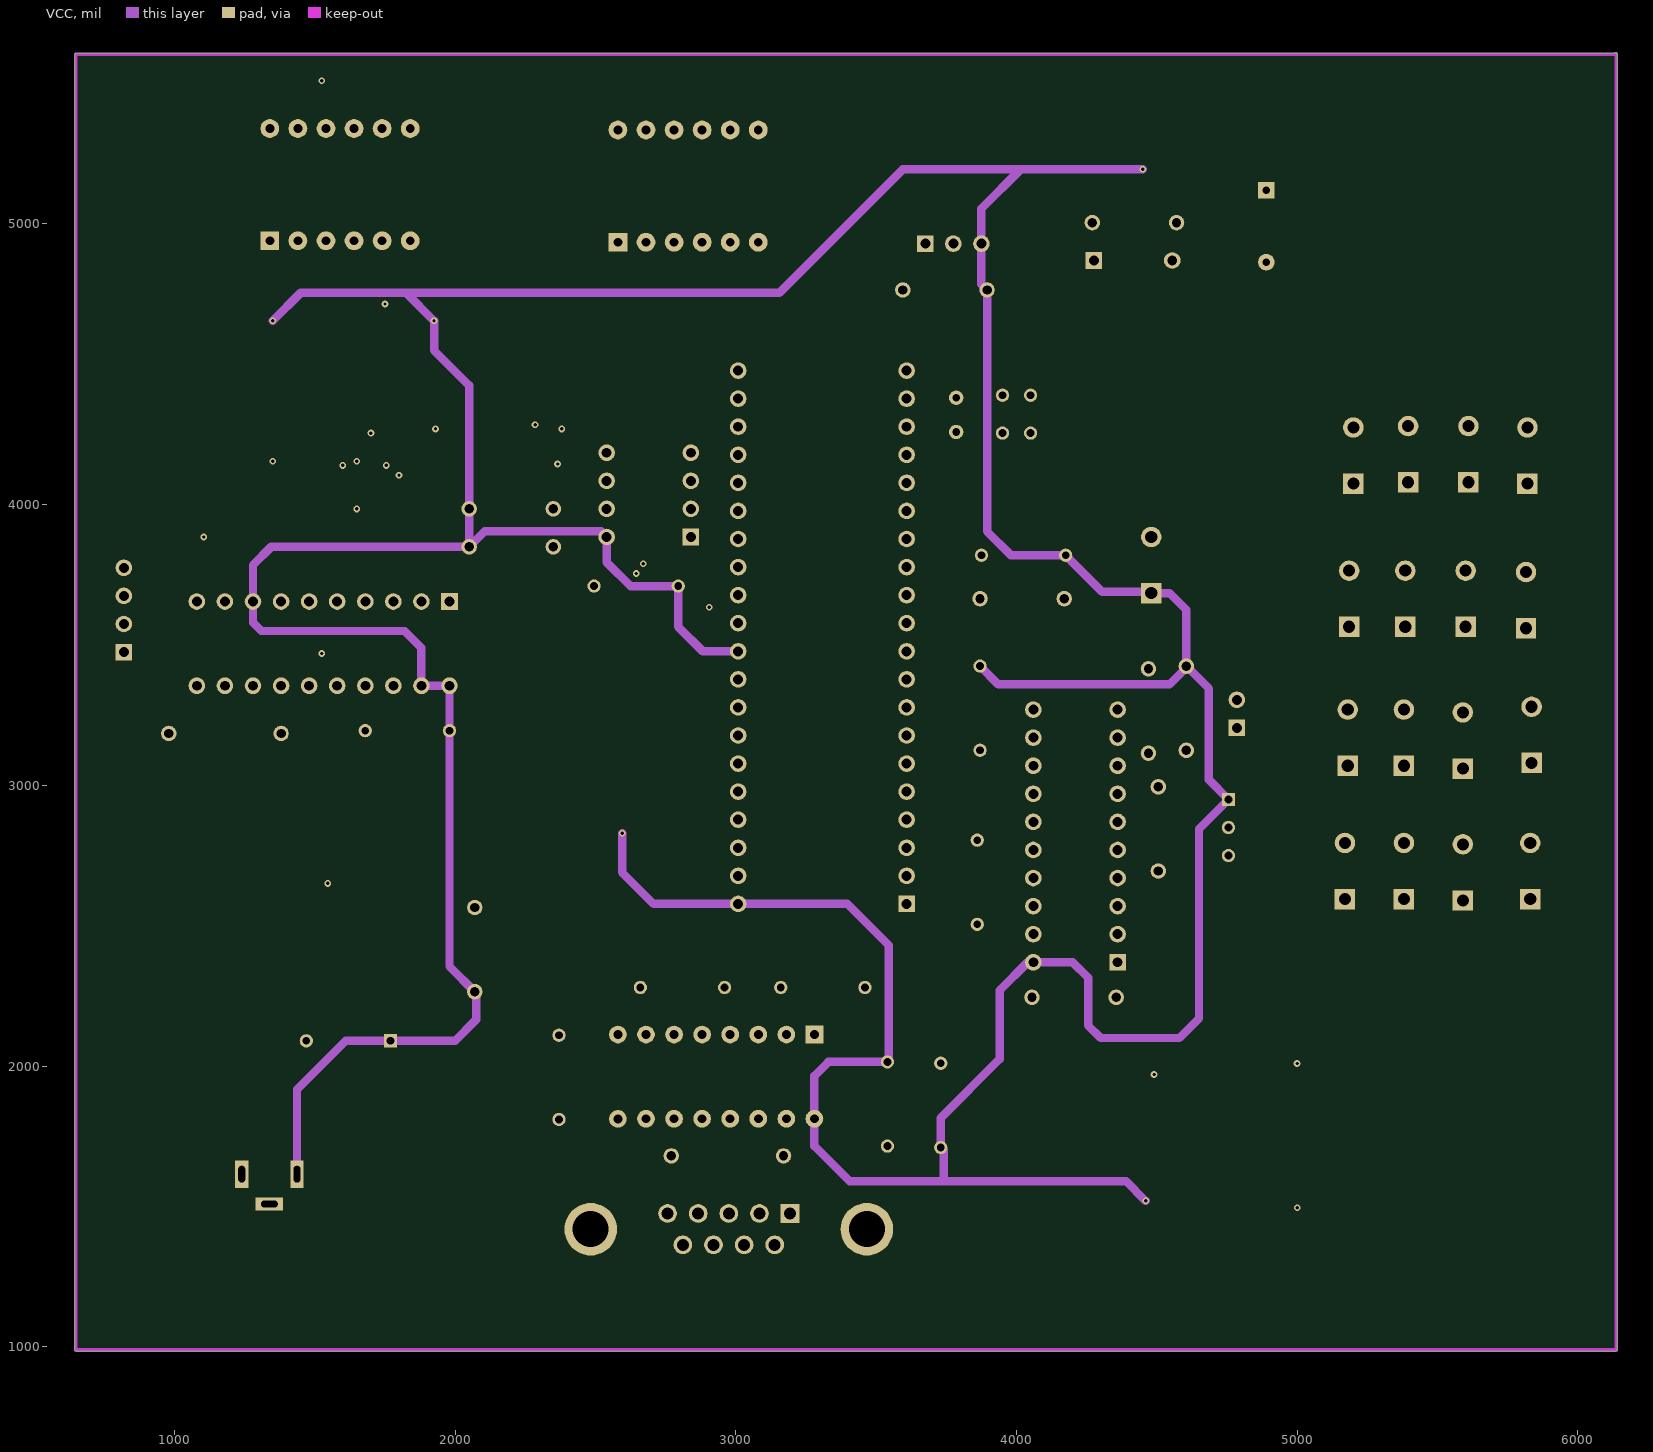
[diagram p0: VCC]
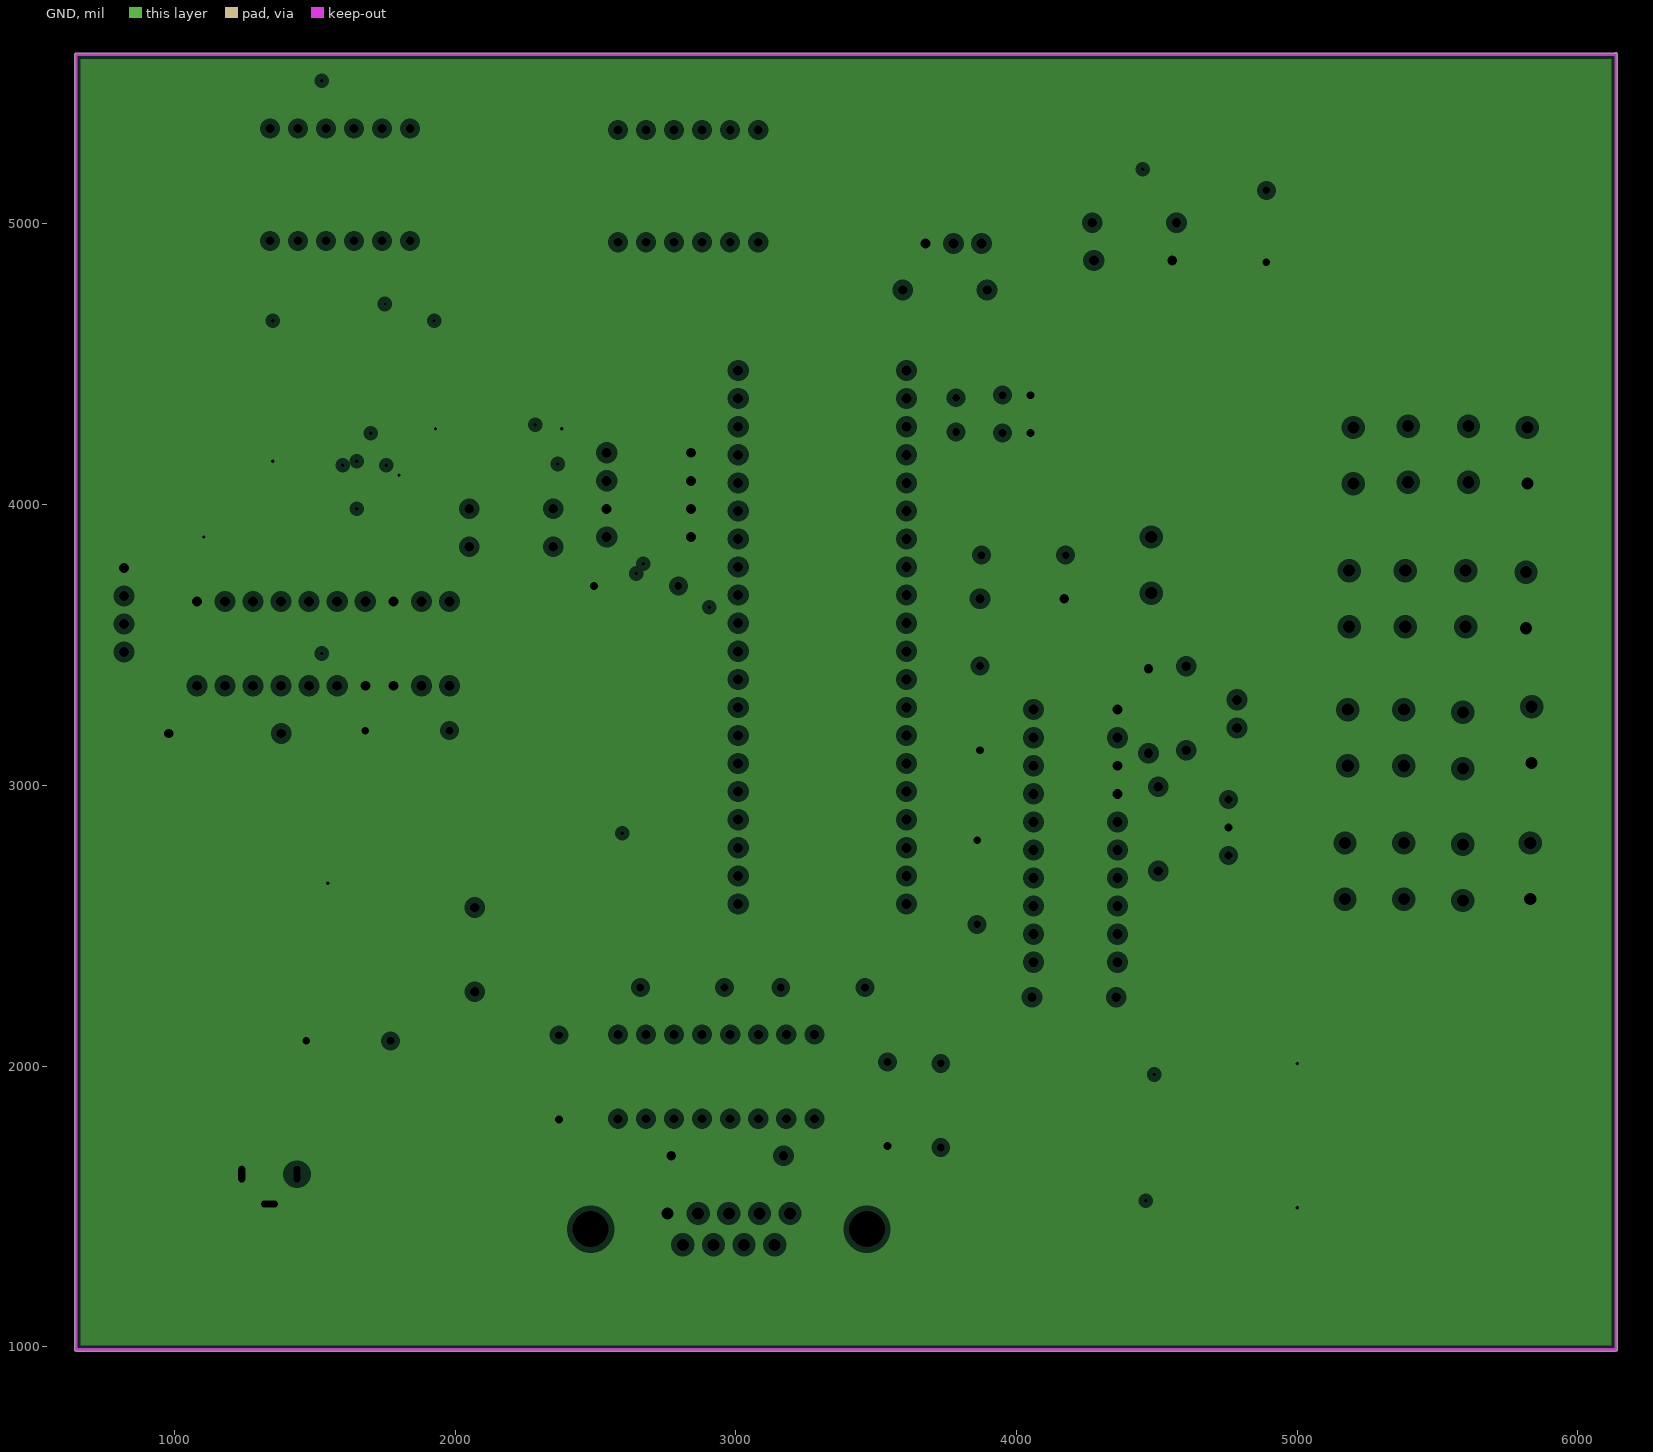
[diagram p1: GND, clearances drawn from the general rule]
# Altium PCB MISC82251.PcbDoc (part 2 of 2)
## Nets (pads, with @x,y where several pads share a name; then routed paths per layer and width w, separated by ;. In a path a pad name is that pad's centre, name@x,y a point inside that pad or via, vN(x,y) a via of type N, cw(c..) or ccw(c..) an arc to the next point about the centre after c; other vN are vias at no path point) (continued)
D0: R8.1 U3.2 U4.2 U5.39 U6.7 | length 3957.8
  Top Layer w10: U4.2 1980,4345 1950,4375 1425,4375 1400,4350 U3.2 1400,3675 U6.7 1380,3445 1430,3395 1430,2990 1645,2775 2620,2775 2705,2860 R8.1 2855,2860 2895,2820 2895,2730 2947.24,2677.76 U5.39
D1: R8.2 U3.3 U4.3 U5.38 U6.6 | length 3717.6
  Top Layer w10: U4.3 2030,4145 2005,4120 1915,4120 1890,4145 1890,4295 1845,4340 1475,4340 1450,4315 U3.3 1450,3685 U6.6 1480,3570 1555,3495 2496.72,3495 2655,3336.72 2655,2970 2715,2910 R8.2 2915,2910 2940,2885 2940,2810 2965,2785 3001.28,2785 U5.38
D2: R8.3 U3.4 U4.4 U5.37 U6.5 | length 3529.2
  Top Layer w10: U4.4 2080,4140 2035,4095 1911.72,4095 1865,4141.72 1865,4290 1845,4310 1525,4310 1500,4285 U3.4 1500,3735 U6.5 1580,3565 1630,3515 2505,3515 2675,3345 2675,2990 2705,2960 R8.3 2926.28,2960 U5.37
D3: R8.4 U3.5 U4.5 U5.36 U6.4 | length 3365.6
  Top Layer w10: U4.5 2130,4135 2065,4070 1895,4070 1845,4120 1845,4270 1830,4285 1570,4285 1550,4265 U3.5 1550,3785 U6.4 1680,3610 1745,3545 2520,3545 2695,3370 2695,3030 2715,3010 R8.4 2976.28,3010 U5.36
D4: R8.5 U3.6 U4.6 U5.35 U6.16 | length 3550.8
  Top Layer w10: v1(1525,3470) 1525,3455 1580,3400 U6.16 ; U3.6 v1(1600,4140) 1700,4040 2115,4040 2180,4105 U4.6 ; R8.5 2990.77,3060 U5.35
  Bottom Layer w10: v1(1525,3470) 1525,4065 v1(1600,4140) ; U6.16 1580,3170 1672.24,3077.76 U5.35
D5: R8.6 U3.7 U4.7 U5.34 U6.15 | length 3531.8
  Top Layer w10: v1(1650,3985) 1690,3945 2029.81,3945 2032.37,3942.44 2132.44,3942.44 2230,4040 U4.7 ; v1(1650,4155) U3.7 ; R8.6 2870,3110 2937.76,3177.76 U5.34
  Bottom Layer w10: U6.15 1480,3375 1535,3430 1635,3430 ; v1(1650,4155) v1(1650,3985) 1650,3725 1630,3705 1630,3435 1635,3430 ; U5.34 2756.28,3430 1635,3430
D6: R8.7 U3.8 U4.8 U5.33 U6.14 | length 4326.4
  Top Layer w10: v1(2285,4285) 2280,4280 U4.8 2280,3810 2455,3635 2625,3635 2715,3545 2715,3204.56 2759.56,3160 R8.7 2850,3160 2875,3185 2875,3230 2922.76,3277.76 U5.33
  Bottom Layer w10: U6.14 1380,3475 1360,3495 1080,3495 1010,3565 1010,4235 1085,4310 1720,4310 ; v1(1700,4255) 1700,4290 1720,4310 ; v1(2285,4285) 2260,4310 1720,4310
D7: R8.8 U3.9 U4.9 U5.32 U6.13 | length 3811.7
  Top Layer w10: U3.9 1750,4145 v1(1755,4140) ; U4.9 2330,4180 v1(2365,4145) 2420,4090 2420,3705 2470,3655 2685,3655 2778.98,3561.02 R8.8 2835,3210 2855,3230 2855,3360 2872.76,3377.76 U5.32
  Bottom Layer w10: U6.13 1280,3295 1300,3275 1415,3275 1430,3290 1430,4115 1515,4200 1705,4200 1755,4150 v1(1755,4140) 2360,4140 v1(2365,4145)
DB1: U2.18 U5.1 U8.19 | length 1908.2
  Top Layer w10: U5.1 4052.24,2577.76 U2.18 4120,2510 4120,1690 4235,1575 U8.19
DB2: U2.17 U5.2 U8.18 | length 1931.8
  Top Layer w10: U5.2 4052.24,2677.76 U2.17 4140,2590 4140,1765 4280,1625 U8.18
DB3: U2.16 U5.3 U8.17 | length 2044.1
  Top Layer w10: U5.3 3631.28,2755 4045,2755 U2.16 4145,2770 4165,2750 4165,1790 4280,1675 U8.17
DB4: U2.15 U5.4 U8.16 | length 2081.6
  Top Layer w10: U5.4 4052.24,2877.76 U2.15 4150,2870 4185,2835 4185,1825 4285,1725 U8.16
DB5: U2.14 U5.5 U8.15 | length 2140.4
  Top Layer w10: U5.5 3616.28,2970 U2.14 4180,2970 4205,2945 4205,1870 4300,1775 U8.15
DB6: U2.13 U5.6 U8.14 | length 2146.5
  Top Layer w10: U5.6 4052.24,3077.76 U2.13 4190,3070 4225,3035 4225,1985 4385,1825 U8.14
DB7: U2.12 U5.7 U8.13 | length 2214.1
  Top Layer w10: U5.7 3616.28,3170 U2.12 4220,3170 4245,3145 4245,2015 4385,1875 U8.13
DB8: U2.11 U5.8 U8.12 | length 2255.3
  Top Layer w10: U5.8 4052.24,3277.76 U2.11 4215,3270 4285,3200 4285,2035 4395,1925 U8.12
DCDEN: U5.14
DIOLA: U5.26 U8.11 | length 3427.4
  Top Layer w10: v1(4490,1970) 4495,1975 U8.11
  Bottom Layer w10: U5.26 3242.24,3977.76 3315,3905 3315,2415 3385,2345 3780,2345 3840,2285 3840,2100 3895,2045 4415,2045 v1(4490,1970)
DP: SMG1.3 SMG2.3 U3.12 | length 2007.4
  Top Layer w10: U3.12 v1(1750,4715)
  Bottom Layer w10: v1(1750,4715) 1750,4775 1715,4810 1575,4810 1540,4845 SMG1.3 1540,4990 1605,5055 2175,5055 2390,4840 2755,4840 2780,4865 SMG2.3
DULA: U3.11 U5.27 | length 1981.3
  Top Layer w10: U3.11 1800,4475 1850,4425 2615,4425 2655,4385 2655,3805 v1(2670,3790)
  Bottom Layer w10: v1(2670,3790) 2920.77,3790 U5.27
E: SMG1.1 SMG2.1 U3.15 | length 2088.7
  Top Layer w10: SMG1.1 1340,4795 1360,4775 1535,4775 1600,4710 U3.15
  Bottom Layer w10: SMG1.1 1340,5075 1375,5110 2515,5110 2580,5045 SMG2.1
F: SMG1.10 SMG2.10 U3.14 | length 4045
  Top Layer w10: v1(1525,5510) 1055,5510 975,5430 975,4545 1045,4475 1605,4475 1650,4520 U3.14
  Bottom Layer w10: v1(1525,5510) 1540,5495 SMG1.10 1540,5260 1575,5225 2415,5225 2450,5260 2450,5420 2480,5450 2735,5450 2780,5405 SMG2.10
G: SMG1.5 SMG2.5 U3.13 | length 1863.2
  Top Layer w10: U3.13 1700,4900 SMG1.5
  Bottom Layer w10: SMG1.5 1805,5005 2125,5005 2350,4780 2945,4780 2980,4815 SMG2.5
GND: C1.1 C4.1 C5.2 C7.1 C8.2 C10.2 C11.2 C12.2 C13.2 D1.2 D2.2 D3.1 J1.5 J2.2 J2.3 LS1.2 LS1.2A P1.1 P3.4 R1.2 R5.1 R7.2 R9.2 R10.1 S2.1 S7.1 S12.1 S17.1 U2.7 U2.8 U2.10 U3.1 U3.10 U4.1 U4.10 U6.3 U6.10 U6.17 U6.18 U7.1 U7.2 U7.3 U7.4 U7.7 U8.1 U8.10 | length 535
  Top Layer w30: D1.2 1099.06,3879.06 v1(1105,3885) ; v1(1350,4155) U3.1 ; D2.2 v1(1545.94,2650.94) v1@1550,2655 ; v1(1800,4105) U3.10 ; U4.1 v1(1930,4270) ; U4.10 v1@2380,4275 ; U8.1 4998.98,1496.02 v1(5000,1495) ; U8.10 4998.98,2008.98 v1@5000,2010
  other v1: 4999.49,2009.49 2380,4270
INT0: S13.1 S14.1 S15.1 S16.1 U5.12 U6.1 | length 5741.9
  Top Layer w10: v1(2905,3635) 2906.77,3633.23 3564,3633.23 U5.12 ; S13.1 5695,2695 5695,2970 ; S14.1 5680,2970 5695,2970 ; S15.1 5685,3565 5695,3555 ; S16.1 5695,3995 5695,3555 ; 5695,2970 5695,3555
  Bottom Layer w10: U6.1 2885,3655 v1(2905,3635) ; U5.12 4140.77,4210 5480,4210 S16.1
INT1: U5.13
LCDEN: S2.2 S3.2 S8.2 S13.2 | length 660
  Bottom Layer w10: S3.2 S8.2 S2.2
M11: SMG1.12 U4.19 | length 1345.2
  Top Layer w10: SMG1.12 1340,5150 1380,5110 1940,5110 1980,5070 U4.19
M12: SMG1.9 U4.18 | length 1048.3
  Top Layer w10: SMG1.9 1640,5230 1715,5155 1945,5155 2030,5070 U4.18
M13: SMG1.8 U4.17 | length 1033.5
  Top Layer w10: SMG1.8 1740,5255 1810,5185 2050,5185 2080,5155 U4.17
M21: SMG2.12 U4.16 | length 1138.5
  Top Layer w10: U4.16 2130,5070 2190,5130 2540,5130 2580,5170 SMG2.12
M22: SMG2.9 U4.15 | length 1385.5
  Top Layer w10: U4.15 2180,5020 2240,5080 2835,5080 2880,5125 SMG2.9
M23: SMG2.8 U4.14 | length 1435.5
  Top Layer w10: U4.14 2230,5015 2275,5060 2920,5060 2980,5120 SMG2.8
NetC2_1: C2.1 U1.1 | length 329.9
  Top Layer w10: U1.1 3280,2250 3310,2280 C2.1
NetC2_2: C2.2 U1.3 | length 200.6
  Top Layer w10: U1.3 3080,2200 C2.2
NetC3_2: C3.2 U1.2 | length 725.6
  Top Layer w10: U1.2 3180,2010 3220,1970 3710,1970 3750,2010 C3.2
NetC5_1: C5.1 R2.1 U2.19 | length 664.4
  Top Layer w10: R2.1 3890,2245 3845,2290 3845,2490 C5.1 4025,2505 U2.19
NetC6_1: C6.1 U1.4 | length 220.7
  Top Layer w10: C6.1 2960,2110 2979.99,2090.01 U1.4
NetC6_2: C6.2 U1.5 | length 331.9
  Top Layer w10: C6.2 2785,2280 2880,2185 U1.5
NetC7_2: C7.2 U1.6 | length 567.2
  Top Layer w10: C7.2 2370,2165 2430,2225 2720,2225 2780,2165 U1.6
NetD1_1: D1.1 P3.3 | length 225.6
  Top Layer w10: P3.3 924.06,3675 D1.1
NetD2_1: D2.1 R12.1 | length 408
  Top Layer w10: D2.1 2065,2570 R12.1
NetD3_2: D3.2 LS1.1 LS1.1A Q1.1 | length 1012.1
  Top Layer w10: D3.2 4345,4870 4377.6,4902.6 Q1.1 4377.6,5242.6 4410,5275 4848.78,5275 LS1.1
NetD4_1: D4.1 R15.8 | length 222.1
  Top Layer w10: D4.1 5723.11,1455 R15.8
NetD4_2: D4.2 U8.2 | length 673.3
  Top Layer w10: U8.2 5080,1575 5110,1545 5110,1430 5170,1370 D4.2
NetD5_1: D5.1 R15.7 | length 485.7
  Top Layer w10: D5.1 5685,1455 5735,1505 R15.7
NetD5_2: D5.2 U8.3 | length 386.6
  Top Layer w10: U8.3 5115,1625 5145,1595 5145,1470 5160,1455 D5.2
NetD6_1: D6.1 R15.6 | length 187.1
  Top Layer w10: D6.1 5645,1555 R15.6
NetD6_2: D6.2 U8.4 | length 624.5
  Top Layer w10: U8.4 5140,1675 5165,1650 5165,1565 5180,1550 D6.2
NetD7_1: D7.1 R15.5 | length 479.5
  Top Layer w10: D7.1 5685,1640 5715,1610 5820,1610 R15.5
NetD7_2: D7.2 U8.5 | length 278.1
  Top Layer w10: U8.5 5156.72,1725 5241.72,1640 D7.2
NetD8_1: D8.1 R15.4 | length 213
  Top Layer w10: D8.1 5718.11,1655 R15.4
NetD8_2: D8.2 U8.6 | length 544.7
  Top Layer w10: U8.6 5135,1775 5180,1730 D8.2
NetD9_1: D9.1 R15.3 | length 512.6
  Top Layer w10: D9.1 5665,1820 5780,1705 R15.3
NetD9_2: D9.2 U8.7 | length 245
  Top Layer w10: U8.7 5236.89,1825 D9.2
NetD10_1: D10.1 R15.2 | length 306.7
  Top Layer w10: D10.1 5730,1910 5750,1890 5750,1785 5780,1755 R15.2
NetD10_2: D10.2 U8.8 | length 541.5
  Top Layer w10: U8.8 5185,1875 5220,1910 D10.2
NetD11_1: D11.1 R15.1 | length 669.9
  Top Layer w10: D11.1 5385,2020 5790,2020 5825,1985 R15.1
NetD11_2: D11.2 U8.9 | length 271.9
  Top Layer w10: U8.9 5171.89,1925 D11.2
NetJ1_2: J1.2 U1.14 | length 339.2
  Top Layer w10: U1.14 3080,1479.06 J1.2
NetJ1_3: J1.3 U1.13 | length 339.6
  Top Layer w10: J1.3 2975,1807.5 U1.13
NetP2_1: P2.1 R4.1 R6.2 R7.1 U2.9 | length 619.6
  Top Layer w10: U2.9 4415,3170 R7.1 ; R4.1 4470,3030 R7.1 ; P2.1 4705,3125 R6.2 4595,3115 R7.1
NetP2_2: P2.2 R1.3 | length 804
  Top Layer w10: R1.3 4885,2750 4915,2780 4915,3265 4875,3305 P2.2
NetP3_1: P3.1 U6.9 | length 517.8
  Top Layer w10: P3.1 1135,3475 1185,3525 1185,3650 U6.9
NetP3_2: P3.2 U6.11 | length 563.8
  Top Layer w10: P3.2 740,3495 740,3405 790,3355 U6.11
NetQ1_2: Q1.2 R11.1 | length 196.3
  Top Layer w10: Q1.2 4452.4,5042.6 4480,5015 4560,5015 R11.1
NetR2_2: R2.2 U2.4 | length 460.2
  Top Layer w10: R2.2 4315,2285 4315,2625 U2.4
NetR4_2: R4.2 U2.6 | length 302.4
  Top Layer w10: U2.6 4475,2870 4505,2840 R4.2
NetR5_2: R5.2 U1.15 | length 136.6
  Top Layer w10: R5.2 3180,1690 U1.15
NetR9_1: R9.1 U6.12 | length 334.9
  Top Layer w10: U6.12 1180,3245 1240,3185 R9.1
P30: S3.1 S4.1 S5.1 S6.1 U1.12 U5.10 | length 7202
  Top Layer w10: U1.12 2879.99,1945.01 2820,2005 2375,2005 2290,2090 2290,2310 2365,2385 3225,2385 3310,2470 3310,3385 3402.76,3477.76 U5.10 ; S3.1 5300,2725 5300,3070 ; S4.1 5300,3070 ; S5.1 5290,3565 5300,3555 ; S6.1 5300,3975 5300,3555 ; 5300,3070 5300,3555
  Bottom Layer w10: U5.10 4592.76,3477.76 4775,3660 4775,4015 4835,4075 S6.1
P31: S8.1 S9.1 S10.1 S11.1 U1.11 U5.11 | length 7603.6
  Top Layer w10: U1.11 2780,1885 2720,1945 2320,1945 2235,2030 2235,2360 2310,2435 3105,2435 3175,2505 3175,3470 3282.76,3577.76 U5.11 ; S8.1 5505,2720 5505,3075 ; S9.1 5500,3070 5505,3075 ; S10.1 5505,3565 ; S11.1 5505,3970 5505,3565 ; 5505,3075 5505,3565
  Bottom Layer w10: U5.11 4562.76,3577.76 4685,3700 4685,4120 4745,4180 5295,4180 S11.1
PSEN: U5.29
RD: S6.2 S11.2 S16.2 S17.2 U2.2 U5.17 | length 5460.9
  Top Layer w10: U5.17 5102.76,4177.76 S6.2 5760,4275 5765,4280 5815,4280 S17.2
  Bottom Layer w10: U5.17 3537.76,4177.76 3430,4070 3430,2460 3455,2435 3875,2435 3930,2380 3930,2255 4020,2165 4185,2165 4215,2195 4215,2400 4285,2470 U2.2
RS: S4.2 S7.2 S9.2 S14.2 U5.15 | length 2743.4
  Top Layer w10: U5.15 4757.24,3977.76 5045,3690 5045,3315 5090,3270 S4.2
  Bottom Layer w10: S4.2 S9.2 5825,3270 S7.2
RST: C9.1 R10.2 S1.2 U5.9 | length 1248.5
  Top Layer w10: U5.9 3717.76,3377.76 3870,3530 R10.2 3870,3815 C9.1 3940,3885 S1.2
SCL: R13.1 U5.22 U7.6 | length 903.5
  Bottom Layer w10: R13.1 2440,3940 2440,3985 U7.6 2832.76,4377.76 U5.22
SDA: R14.1 U5.21 U7.5 | length 1009.1
  Bottom Layer w10: R14.1 2455,4090 2455,4100 U7.5 2540,4425 2592.76,4477.76 U5.21
SPK: R11.2 U5.24 | length 1899.9
  Bottom Layer w10: U5.24 3307.76,4177.76 3430,4300 3430,4590 3490,4650 4045,4650 4135,4740 4135,4955 4185,5005 R11.2
VCC: C1.2 C3.1 C4.2 C8.1 C9.2 C10.1 C12.1 J2.1 P1.3 Q1.3 R1.1 R3.2 R6.1 R8.9 R8.10 R8.11 R8.12 R8.13 R8.14 R8.15 R8.16 R12.2 R13.2 R14.2 R15.9 R15.10 R15.11 R15.12 R15.13 R15.14 R15.15 R15.16 S1.1 U1.16 U2.20 U3.20 U4.20 U5.31 U5.40 U6.8 U6.19 U6.20 U7.8 U8.20 | length 22354.1
  Top Layer w30: U3.20 v1(1350,4655) ; v1(1925,4655) 1930,4650 U4.20 ; R8.9 R8.10 R8.11 R8.12 R8.13 R8.14 R8.15 R8.16 2590,2835 v1(2595,2830) ; Q1.3 4449.29,5194.29 v1(4450,5195) ; v1(4460,1520) 4465,1525 U8.20 4621.02,1343.98 4755,1210 5920,1210 6013.98,1303.98 R15.9 R15.10 R15.11 R15.12 R15.13 R15.14 R15.15 R15.16
  VCC w30: v1(1350,4655) 1450,4755 1825,4755 ; J2.1 1436.85,1916.85 1610,2090 C10.1 2000,2090 2075,2165 2075,2260 R12.2 1980,2355 C8.1 U6.20 U6.19 1880,3490 1820,3550 1310,3550 1280,3580 U6.8 1280,3785 1345,3850 R13.2 ; v1(2595,2830) 2595,2690 2707.24,2577.76 U5.40 3397.24,2577.76 3545,2430 3545,2020 C4.2 3329.99,2015 3279.99,1965 U1.16 3279.99,1715.01 3405,1590 3740,1590 ; U5.31 2882.24,3477.76 2795,3565 C12.1 2625,3710 2540,3795 U7.8 2520,3905 2105,3905 R13.2 ; C1.2 3935,3360 4545,3360 4605,3420 R6.1 ; v1(4450,5195) 4015,5195 ; v1(4460,1520) 4390,1590 3740,1590 ; 1825,4755 3155,4755 3595,5195 4015,5195 ; 1825,4755 v1(1925,4655) 1925,4550 2050,4425 R14.2 R13.2 ; 3740,1590 3740,1700 C3.1 3730,1815 3940,2025 3940,2270 4040,2370 U2.20 4200,2370 4255,2315 4255,2145 4300,2100 4580,2100 4650,2170 4650,2845 R1.1 4685,3020 4685,3345 R6.1 ; 4015,5195 3875,5055 P1.3 3875,4785 R3.2 3895,3905 3980,3820 C9.2 4305,3690 4475,3690 S1.1 4545,3685 4605,3625 R6.1
WELA: U4.11 U5.28 | length 1380
  Top Layer w10: U4.11 2662.05,4587.95 2695,4555 2695,3845 2762.24,3777.76 U5.28
WR: S5.2 S10.2 S12.2 S15.2 U2.3 U5.16 U6.2 | length 7251
  Top Layer w10: v1(2645,3755) 2915,3755 2940,3730 3075,3730 3422.76,4077.76 U5.16 4762.24,4077.76 5075,3765 S5.2 ; U2.3 4965,2570 5045,2490 5890,2490 5980,2580 5980,3680 5905,3755 5820,3755 S12.2
  Bottom Layer w10: U6.2 1980,3755 v1(2645,3755) ; S5.2 S10.2 S15.2 5810,3765 S12.2
XTAL1: C11.1 U5.19 Y1.2 | length 346.5
  Top Layer w10: U5.19 3781.73,4377.76 Y1.2 3941.02,4381.02 C11.1
XTAL2: C13.1 U5.18 Y1.1 | length 350.9
  Top Layer w10: U5.18 3766.22,4277.76 Y1.1 3946.02,4258.98 C13.1
pads on no net: J1.1 J1.4 J1.6 J1.7 J1.8 J1.9 J1.10 J1.11 SMG1.6 SMG2.6 U1.7 U1.8 U1.9 U1.10 U2.5 U4.12 U4.13 U5.20

## Polygon pours and split planes (outlines as drawn)
GND on GND (split plane): 6119.92,1005.08 665.08,1005.08 665.08,5587.85 6119.92,5587.85

## Keep-outs
Keep-Out Layer:
  lines w10: 650,5325 650,5480 650,5602.93 6120,5602.93 6130,5602.93 ccw(c6130,5610) 6135,5605 6135,5470 ; 650,5375 650,990 6135,990 6135,5480